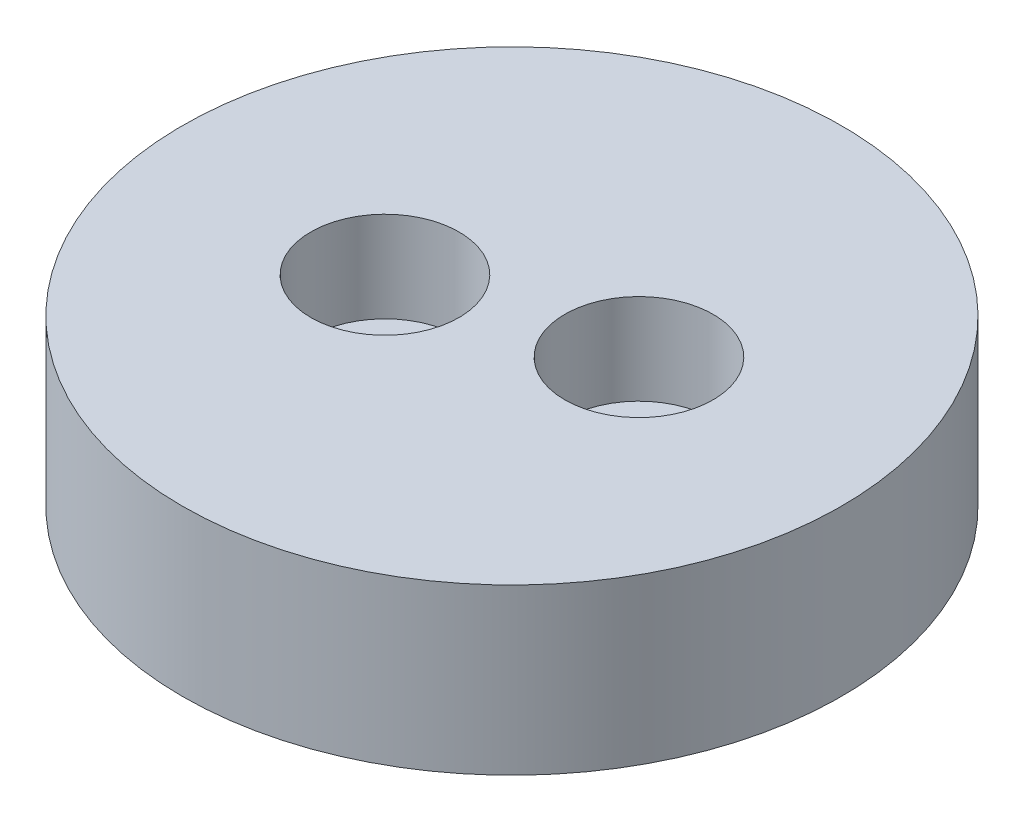
SolidWorks part; units mm, degrees
ref_plane "Front Plane" through (0, 0, 0) normal (0, 0, 1) x (1, 0, 0)
ref_plane "Top Plane" through (0, 0, 0) normal (0, 1, 0) x (1, 0, 0)
ref_plane "Right Plane" through (0, 0, 0) normal (1, 0, 0) x (0, 0, -1)
sketch "Sketch1" plane through (0, 0, 0) normal (0, 1, 0) x (1, 0, 0)
  circle A0 centre (0, 0) radius 40
  dimension "D1" = 80
extrude "Boss-Extrude1" add sketch "Sketch1" along normal blind 20
sketch "Sketch2" plane through (0, 20, 0) normal (0, 1, 0) x (1, 0, 0)
  point P0 (-12.0342, -3.3804)
  point P1 (12.0342, 3.3804)
hole_wizard "Hole size (per socket head cap screw type) 1" positions "3DSketch1" profile "Sketch3" counterbore size "M10" standard "GB" end condition through all
sketch3d "3DSketch1"
  point P0 (-12.0342, 20, 3.3804)
  point P3 (12.0342, 20, -3.3804)
sketch "Sketch3" plane through (-12.0342, 20, 3.3804) normal (1, 0, 0) x (0, 0, 1)
  line L0 (0, 0) -> (0, 20)
  line L1 (0, 20) -> (5.5, 20)
  line L3 (5.5, 20) -> (5.5, 11)
  line L4 (5.5, 11) -> (9, 11)
  line L5 (9, 11) -> (9, 0)
  line L7 (9, 0) -> (0, 0)
  line L11 (0, -6.35) -> (0, 107.95) construction
  dimension "通孔孔直径" = 11
  dimension "通孔孔深度" = 20
  dimension "柱形沉头孔直径" = 18
  dimension "柱形沉头孔深度" = 11
